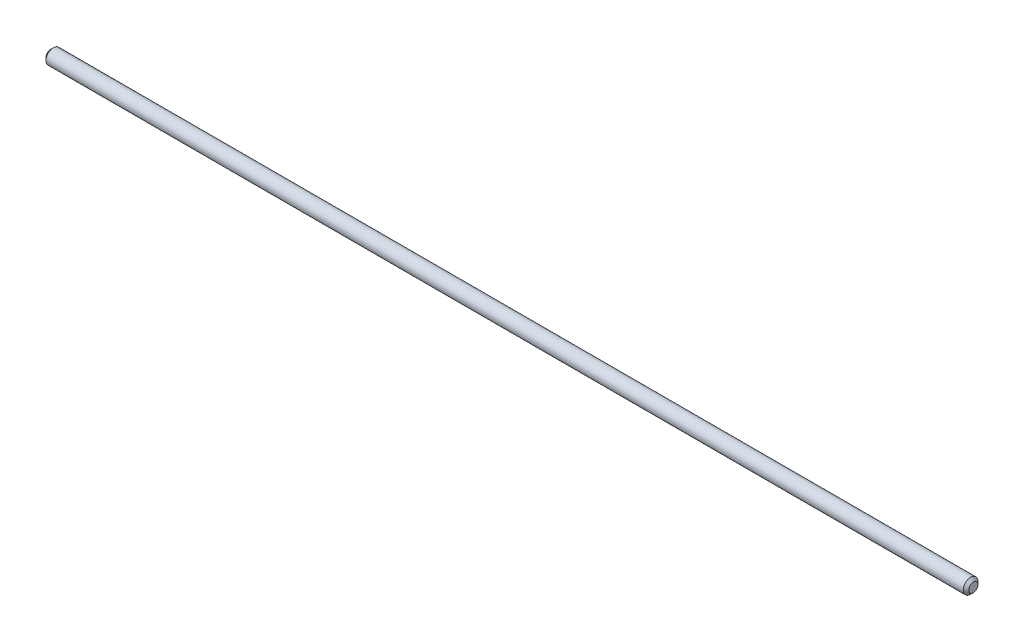
SolidWorks part; units mm, degrees
material "1060 Alloy"
ref_plane "Front Plane" through (0, 0, 0) normal (0, 0, 1) x (1, 0, 0)
ref_plane "Top Plane" through (0, 0, 0) normal (0, 1, 0) x (1, 0, 0)
ref_plane "Right Plane" through (0, 0, 0) normal (1, 0, 0) x (0, 0, -1)
sketch "Sketch1" plane through (0, 0, 0) normal (1, 0, 0) x (0, 0, -1)
  circle A0 centre (0, 0) radius 4
  dimension "D1" = 8
extrude "Boss-Extrude1" add sketch "Sketch1" along normal mid plane 500
chamfer "Chamfer1" distance 1.5 angle 45 2 edges at (-250, 0, -4) (250, 0, -4)
